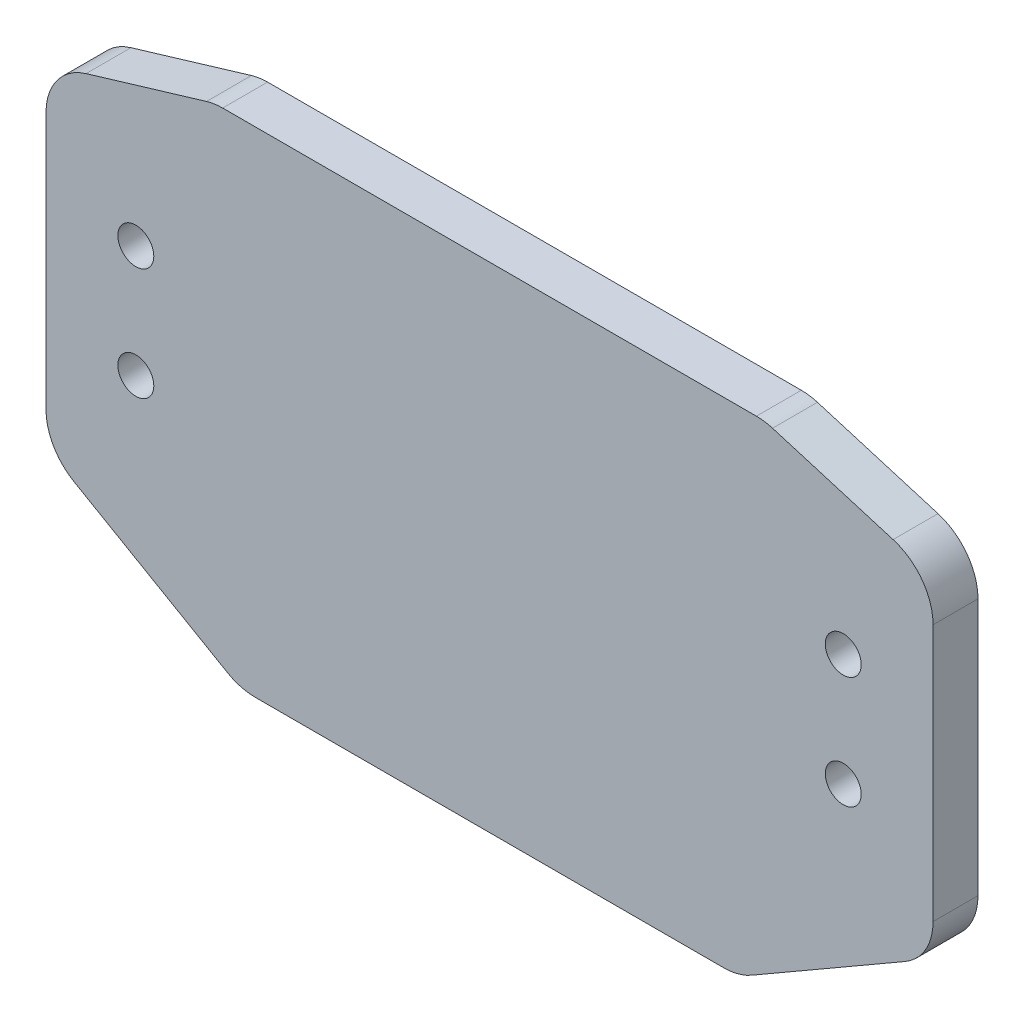
from build123d import *

# Parameters (mm, degrees)
SKETCH1_R           = 1.6
BOSS_EXTRUDE1_DEPTH = 4
R5_FILLET_1_R       = 5


with BuildPart() as part:
    # Sketch1 → Boss-Extrude1 (new body)
    with BuildSketch(Plane.XY):
        Polygon((-24.5, 23.5), (24.5, 23.5), (39.5, 19), (39.5, -10.5), (22.179491924, -20.5), (-22.179491924, -20.5), (-39.5, -10.5), (-39.5, 19), align=None)
        with Locations((-31.5, 9)):
            Circle(SKETCH1_R, mode=Mode.SUBTRACT)
        with Locations((-31.5, -1)):
            Circle(SKETCH1_R, mode=Mode.SUBTRACT)
        with Locations(Location((31.5, -1, 0), (0, 0, 180))):
            Circle(SKETCH1_R, mode=Mode.SUBTRACT)
        with Locations(Location((31.5, 9, 0), (0, 0, 180))):
            Circle(SKETCH1_R, mode=Mode.SUBTRACT)
    extrude(amount=BOSS_EXTRUDE1_DEPTH)

    # R5 Fillet 1
    r5_fillet_1_edges = [part.edges().sort_by_distance(p)[0] for p in [
        (-24.5, 23.5, 2),
        (24.5, 23.5, 2),
        (39.5, 19, 2),
        (39.5, -10.5, 2),
        (22.179491924, -20.5, 2),
        (-22.179491924, -20.5, 2),
        (-39.5, -10.5, 2),
        (-39.5, 19, 2),
    ]]
    fillet(r5_fillet_1_edges, radius=R5_FILLET_1_R)


solid = part.part
